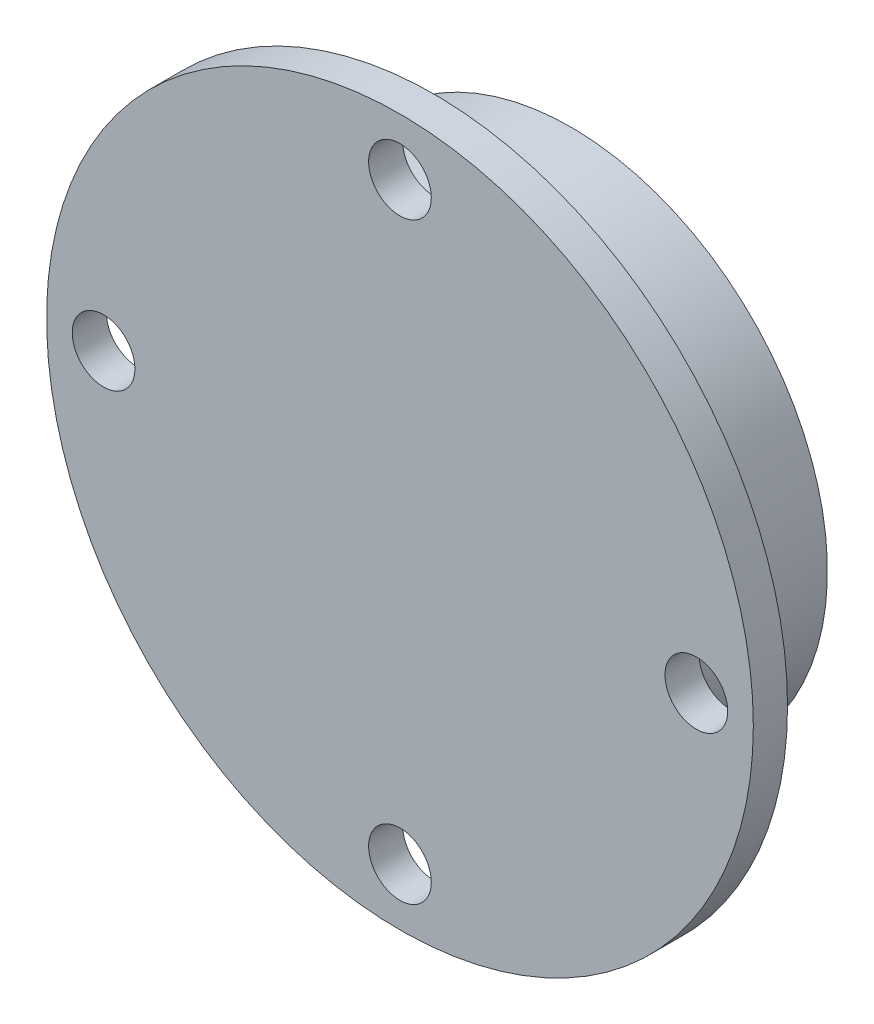
SolidWorks part; units mm, degrees
ref_plane "Front Plane" through (0, 0, 0) normal (0, 0, 1) x (1, 0, 0)
ref_plane "Top Plane" through (0, 0, 0) normal (0, 1, 0) x (1, 0, 0)
ref_plane "Right Plane" through (0, 0, 0) normal (1, 0, 0) x (0, 0, -1)
other "Configuration Table"
sketch "Sketch2" plane through (0, 0, -694.1899) normal (0, 0, 1) x (1, 0, 0)
  circle A0 centre (-50, 0) radius 22.5 construction
  circle A1 centre (-50, 0) radius 31
  dimension "D1" = 62
extrude "Boss-Extrude1" add sketch "Sketch2" along normal blind 3
sketch "Sketch3" plane through (0, 0, -694.1899) normal (0, 0, -1) x (-1, 0, 0)
  circle A0 centre (50, 0) radius 22.5
  dimension "D1" = 45
extrude "Boss-Extrude2" add sketch "Sketch3" along normal blind 12
sketch "Sketch4" plane through (0, 0, -706.1899) normal (0, 0, -1) x (-1, 0, 0)
  circle A0 centre (50, 0) radius 17.5
  dimension "D1" = 35
extrude "Cut-Extrude1" cut sketch "Sketch4" against normal blind 9
sketch "Sketch6" plane through (0, 0, -691.1899) normal (0, 0, 1) x (1, 0, 0)
  circle A0 centre (-50, 0) radius 26 construction
  circle A1 centre (-50, 26) radius 2.75
  circle A2 centre (-24, 0) radius 2.75
  circle A3 centre (-50, -26) radius 2.75
  circle A4 centre (-76, 0) radius 2.75
  dimension "D1" = 52
  dimension "D2" = 5.5
  dimension "D3" = 4
extrude "Cut-Extrude2" cut sketch "Sketch6" against normal blind 12
